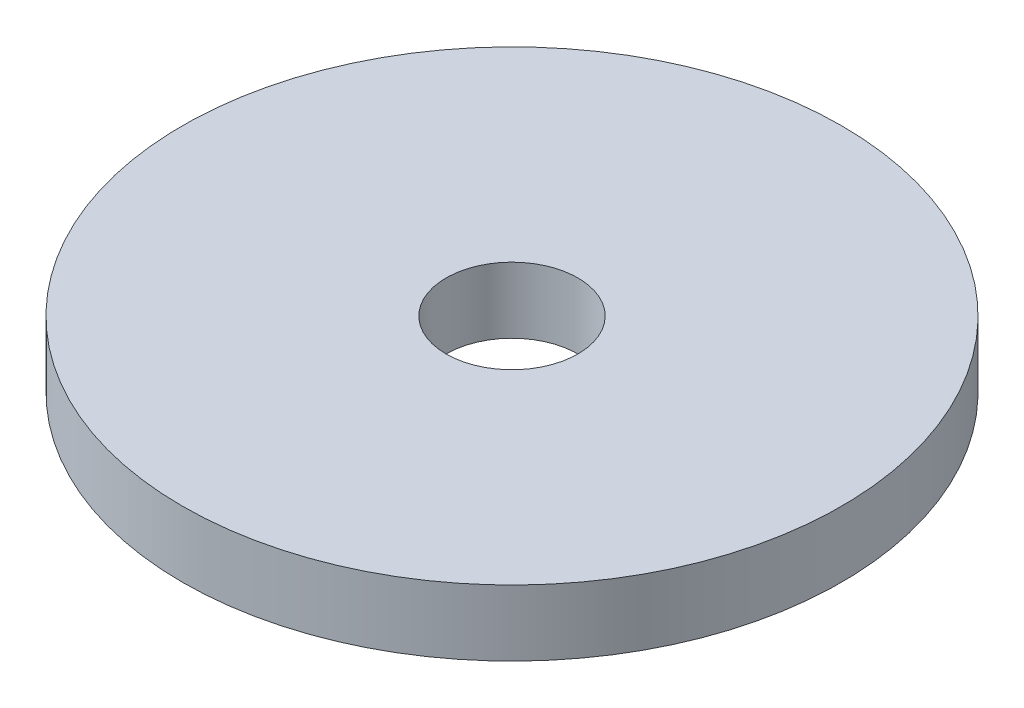
from build123d import *

# Parameters (mm, degrees)
SKETCH1_R           = 10
SKETCH1_R_2         = 2
BOSS_EXTRUDE1_DEPTH = 2


with BuildPart() as part:
    # Sketch1 → Boss-Extrude1 (new body)
    with BuildSketch(Plane(origin=(0, 0, 0), x_dir=(1, 0, 0), z_dir=(0, 1, 0))):
        with Locations(Location((0, 0, 0), (0, 0, 270))):
            Circle(SKETCH1_R)
        with Locations(Location((0, 0, 0), (0, 0, 270))):
            Circle(SKETCH1_R_2, mode=Mode.SUBTRACT)
    extrude(amount=BOSS_EXTRUDE1_DEPTH)


solid = part.part
